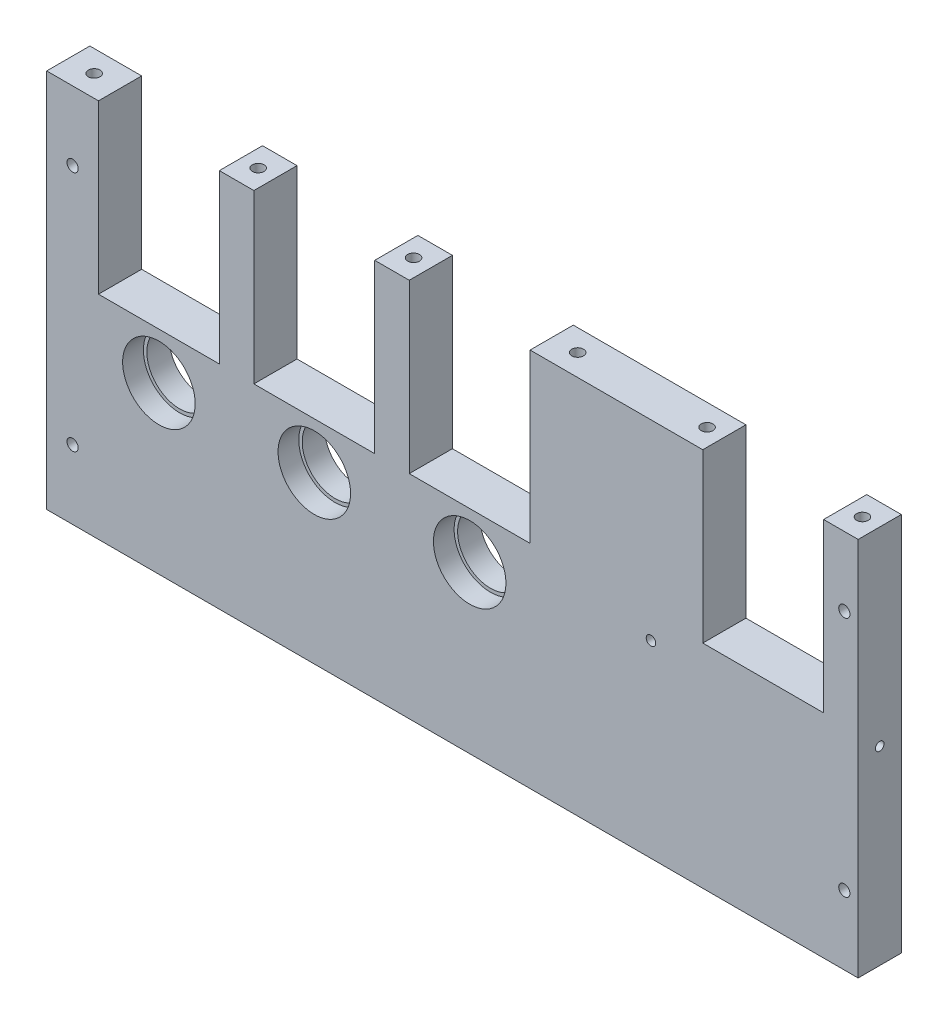
SolidWorks part; units mm, degrees
ref_plane "Front Plane" through (0, 0, 0) normal (0, 0, 1) x (1, 0, 0)
ref_plane "Top Plane" through (0, 0, 0) normal (0, 1, 0) x (1, 0, 0)
ref_plane "Right Plane" through (0, 0, 0) normal (1, 0, 0) x (0, 0, -1)
sketch "Sketch1" plane through (0, 0, 0) normal (0, 0, 1) x (1, 0, 0)
  line L1 (-235, -130) -> (235, -130)
  line L2 (-235, -130) -> (-235, 130)
  line L3 (-235, 130) -> (235, 130)
  line L4 (235, -130) -> (235, 130)
  line L5 (-235, -130) -> (235, 130) construction
  line L6 (-235, 130) -> (235, -130) construction
  point P0 (0, 0)
  dimension "D1" = 470
  dimension "D2" = 260
extrude "Boss-Extrude1" add sketch "Sketch1" along normal mid plane 25
sketch "Sketch4" plane through (0, 0, 12.5) normal (0, 0, 1) x (1, 0, 0)
  line L0 (-205, 130) -> (-205, 33)
  line L1 (235, 130) -> (-235, 130) construction
  line L2 (-205, 33) -> (-135, 33)
  line L3 (-135, 33) -> (-135, 130)
  line L4 (-205, 130) -> (-135, 130)
  line L5 (-115, 130) -> (-115, 33)
  line L6 (-115, 33) -> (-45, 33)
  line L7 (-45, 33) -> (-45, 130)
  line L8 (-25, 130) -> (-25, 33)
  line L9 (-25, 33) -> (45, 33)
  line L10 (45, 33) -> (45, 130)
  line L11 (45, 130) -> (-25, 130)
  line L12 (145, 130) -> (145, 33)
  line L14 (215, 33) -> (215, 130)
  line L15 (215, 130) -> (145, 130)
  line L16 (-235, 130) -> (-235, -130) construction
  line L17 (145, 33) -> (215, 33)
  point P15 (140, 33.5)
  point P17 (210, 33.5)
  point P20 (175, 33.5)
  point P21 (175, -70.6333)
  point P22 (155, 33.5)
  point P23 (155, -70.6333)
  point P24 (195, 33.5)
  point P25 (195, -70.6333)
  point P26 (140, -21.5)
  point P27 (210, -21.5)
  dimension "D1" = 30
  dimension "D2" = 70
  dimension "D3" = 100
  dimension "D4" = 70
  dimension "D7" = 20
  dimension "D8" = 20
  dimension "D9" = 97
extrude "Cut-Extrude3" cut sketch "Sketch4" against normal blind 97
sketch "Sketch5" plane through (0, 0, 12.5) normal (0, 0, 1) x (1, 0, 0)
  line L0 (235, -130) -> (235, 130) construction
  line L1 (-235, -130) -> (235, -130) construction
  circle A0 centre (115, 19.25) radius 2.75
  dimension "D1" = 5.5
  dimension "D2" = 120
  dimension "D3" = 149.25
extrude "Cut-Extrude4" cut sketch "Sketch5" against normal blind 97
sketch "Sketch6" plane through (0, 0, -12.5) normal (0, 0, -1) x (-1, 0, 0)
  circle A0 centre (-115, 19.25) radius 5
  dimension "D1" = 10
extrude "Cut-Extrude5" cut sketch "Sketch6" against normal blind 8
sketch "Sketch7" plane through (0, 0, -12.5) normal (0, 0, -1) x (-1, 0, 0)
  line L0 (235, -130) -> (-235, -130) construction
  line L1 (-271.2617, -90) -> (322.268, -90)
  line L2 (-271.2617, -90) -> (-271.2617, -227.6989)
  line L3 (-271.2617, -227.6989) -> (322.268, -227.6989)
  line L4 (322.268, -90) -> (322.268, -227.6989)
  dimension "D1" = 40
extrude "Cut-Extrude6" cut sketch "Sketch7" against normal blind 40
hole_wizard "M8 Tapped Hole1" positions "Sketch10" profile "Sketch9" tap size "M8" standard "Gb"
sketch "Sketch10" plane through (0, 130, 0) normal (0, 1, 0) x (1, 0, 0)
  line L0 (-235, -12.5) -> (-235, 12.5) construction
  line L1 (-205, 12.5) -> (-235, 12.5) construction
  line L2 (-115, 12.5) -> (-135, 12.5) construction
  line L3 (-25, 12.5) -> (-45, 12.5) construction
  line L4 (145, 12.5) -> (45, 12.5) construction
  line L5 (235, 12.5) -> (215, 12.5) construction
  line L6 (235, -12.5) -> (235, 12.5) construction
  line L8 (-45, 12.5) -> (-45, -12.5) construction
  line L10 (145, 12.5) -> (145, -12.5) construction
  line L11 (45, 12.5) -> (45, -12.5) construction
  point P0 (-220, 0)
  point P2 (225, 0)
  point P4 (135, 0)
  point P6 (-35, 0)
  point P8 (-125, 0)
  point P38 (60, 0)
  dimension "D1" = 15
  dimension "D2" = 12.5
  dimension "D3" = 12.5
  dimension "D4" = 12.5
  dimension "D5" = 12.5
  dimension "D6" = 12.5
  dimension "D7" = 10
  dimension "D8" = 95
  dimension "D9" = 10
  dimension "D10" = 10
  dimension "D11" = 15
  dimension "D12" = 12.5
sketch "Sketch9" plane through (-220, 130, 0) normal (1, 0, 0) x (0, 0, 1)
  line L0 (0, 0) -> (0, 22.0429)
  line L1 (0, 22.0429) -> (3.4, 20)
  line L2 (3.4, 20) -> (3.4, 0)
  line L5 (3.4, 0) -> (0, 0)
  line L10 (0, 22.0429) -> (-3.4, 20) construction
  line L11 (0, -6.35) -> (0, 107.95) construction
  dimension "螺纹孔钻头直径" = 6.8
  dimension "螺纹孔钻头深度" = 20
  dimension "导头角度" = 118
cosmetic thread "Cosmetic Thread1" parameters "D1"=16, "D2"=8
cosmetic thread "Cosmetic Thread2" parameters "D1"=16, "D2"=8
cosmetic thread "Cosmetic Thread3" parameters "D1"=16, "D2"=8
cosmetic thread "Cosmetic Thread4" parameters "D1"=16, "D2"=8
cosmetic thread "Cosmetic Thread5" parameters "D1"=16, "D2"=8
cosmetic thread "Cosmetic Thread8" parameters "D1"=16, "D2"=8
hole_wizard "M10 Tapped Hole1" positions "Sketch12" profile "Sketch11" tap size "M10" standard "Gb"
sketch "Sketch12" plane through (0, -90, 0) normal (0, -1, 0) x (-1, 0, 0)
  line L0 (235, 12.5) -> (-235, 12.5) construction
  line L1 (-235, -12.5) -> (-235, 12.5) construction
  line L2 (235, 12.5) -> (235, -12.5) construction
  point P0 (-155, 0)
  point P2 (155, 0)
  dimension "D1" = 12.5
  dimension "D2" = 80
  dimension "D3" = 80
  dimension "D4" = 12.5
sketch "Sketch11" plane through (155, -90, 0) normal (1, 0, 0) x (0, 0, -1)
  line L0 (0, 0) -> (0, 30.0537)
  line L1 (0, 30.0537) -> (4.25, 27.5)
  line L2 (4.25, 27.5) -> (4.25, 0)
  line L5 (4.25, 0) -> (0, 0)
  line L10 (0, 30.0537) -> (-4.25, 27.5) construction
  line L11 (0, -6.35) -> (0, 107.95) construction
  dimension "螺纹孔钻头直径" = 8.5
  dimension "螺纹孔钻头深度" = 27.5
  dimension "导头角度" = 118
cosmetic thread "Cosmetic Thread6" parameters "D1"=20, "D2"=10
cosmetic thread "Cosmetic Thread7" parameters "D1"=20, "D2"=10
sketch "Sketch13" plane through (0, 0, 12.5) normal (0, 0, 1) x (1, 0, 0)
  line L0 (-205, 33) -> (-135, 33) construction
  line L1 (-205, 130) -> (-205, 33) construction
  circle A0 centre (-170, 6) radius 19
  dimension "D3" = 38
  dimension "D1" = 27
  dimension "D2" = 35
extrude "Cut-Extrude7" cut sketch "Sketch13" against normal through all
sketch "Sketch14" plane through (0, 0, 12.5) normal (0, 0, 1) x (1, 0, 0)
  circle A0 centre (-170, 6) radius 21
  dimension "D1" = 42
extrude "Cut-Extrude8" cut sketch "Sketch14" against normal blind 12
pattern_linear "LPattern1" count 3 spacing 90 along (1, 0, 0) of "Cut-Extrude7", "Cut-Extrude8"
sketch "Sketch15" plane through (0, 0, -12.5) normal (0, 0, -1) x (-1, 0, 0)
  line L0 (-235, -90) -> (-235, 130) construction
  line L1 (-235, 130) -> (-215, 130) construction
  line L2 (235, -90) -> (-235, -90) construction
  circle A0 centre (-227, 90) radius 3.25
  circle A1 centre (-227, -50) radius 3.25
  dimension "D5" = 6.5
  dimension "D1" = 8
  dimension "D2" = 40
  dimension "D3" = 40
  dimension "D4" = 8
extrude "Cut-Extrude9" cut sketch "Sketch15" against normal through all
sketch "Sketch16" plane through (0, 0, -12.5) normal (0, 0, -1) x (-1, 0, 0)
  circle A0 centre (-227, 90) radius 5.5
  circle A1 centre (-227, -50) radius 5.5
  dimension "D1" = 11
extrude "Cut-Extrude10" cut sketch "Sketch16" against normal blind 10
pattern_linear "LPattern2" count 2 spacing 447 along (-1, 0, 0) of "Cut-Extrude9", "Cut-Extrude10"
hole_wizard "M6 Tapped Hole1" positions "3DSketch1" profile "Sketch17" tap size "M6" standard "GB"
sketch3d "3DSketch1"
  line L0 (235, -90, -12.5) -> (235, 130, -12.5) construction
  line L1 (235, -90, 12.5) -> (235, -90, -12.5) construction
  line L2 (-235, 130, -12.5) -> (-235, -90, -12.5) construction
  line L3 (-235, -90, -12.5) -> (-235, -90, 12.5) construction
  point P0 (-235, 20, 0)
  point P2 (235, 20, 0)
  dimension "D1" = 12.5
  dimension "D2" = 110
  dimension "D3" = 12.5
  dimension "D4" = 110
sketch "Sketch17" plane through (-235, 20, 0) normal (0, 1, 0) x (0, 0, 1)
  line L0 (0, 0) -> (0, 16.0022)
  line L1 (0, 16.0022) -> (2.5, 14.5)
  line L2 (2.5, 14.5) -> (2.5, 0)
  line L5 (2.5, 0) -> (0, 0)
  line L10 (0, 16.0022) -> (-2.5, 14.5) construction
  line L11 (0, -6.35) -> (0, 107.95) construction
  dimension "螺纹孔钻头直径" = 5
  dimension "螺纹孔钻头深度" = 14.5
  dimension "导头角度" = 118
cosmetic thread "Cosmetic Thread9" parameters "D1"=11.5, "D2"=6
cosmetic thread "Cosmetic Thread10" parameters "D1"=11.5, "D2"=6
